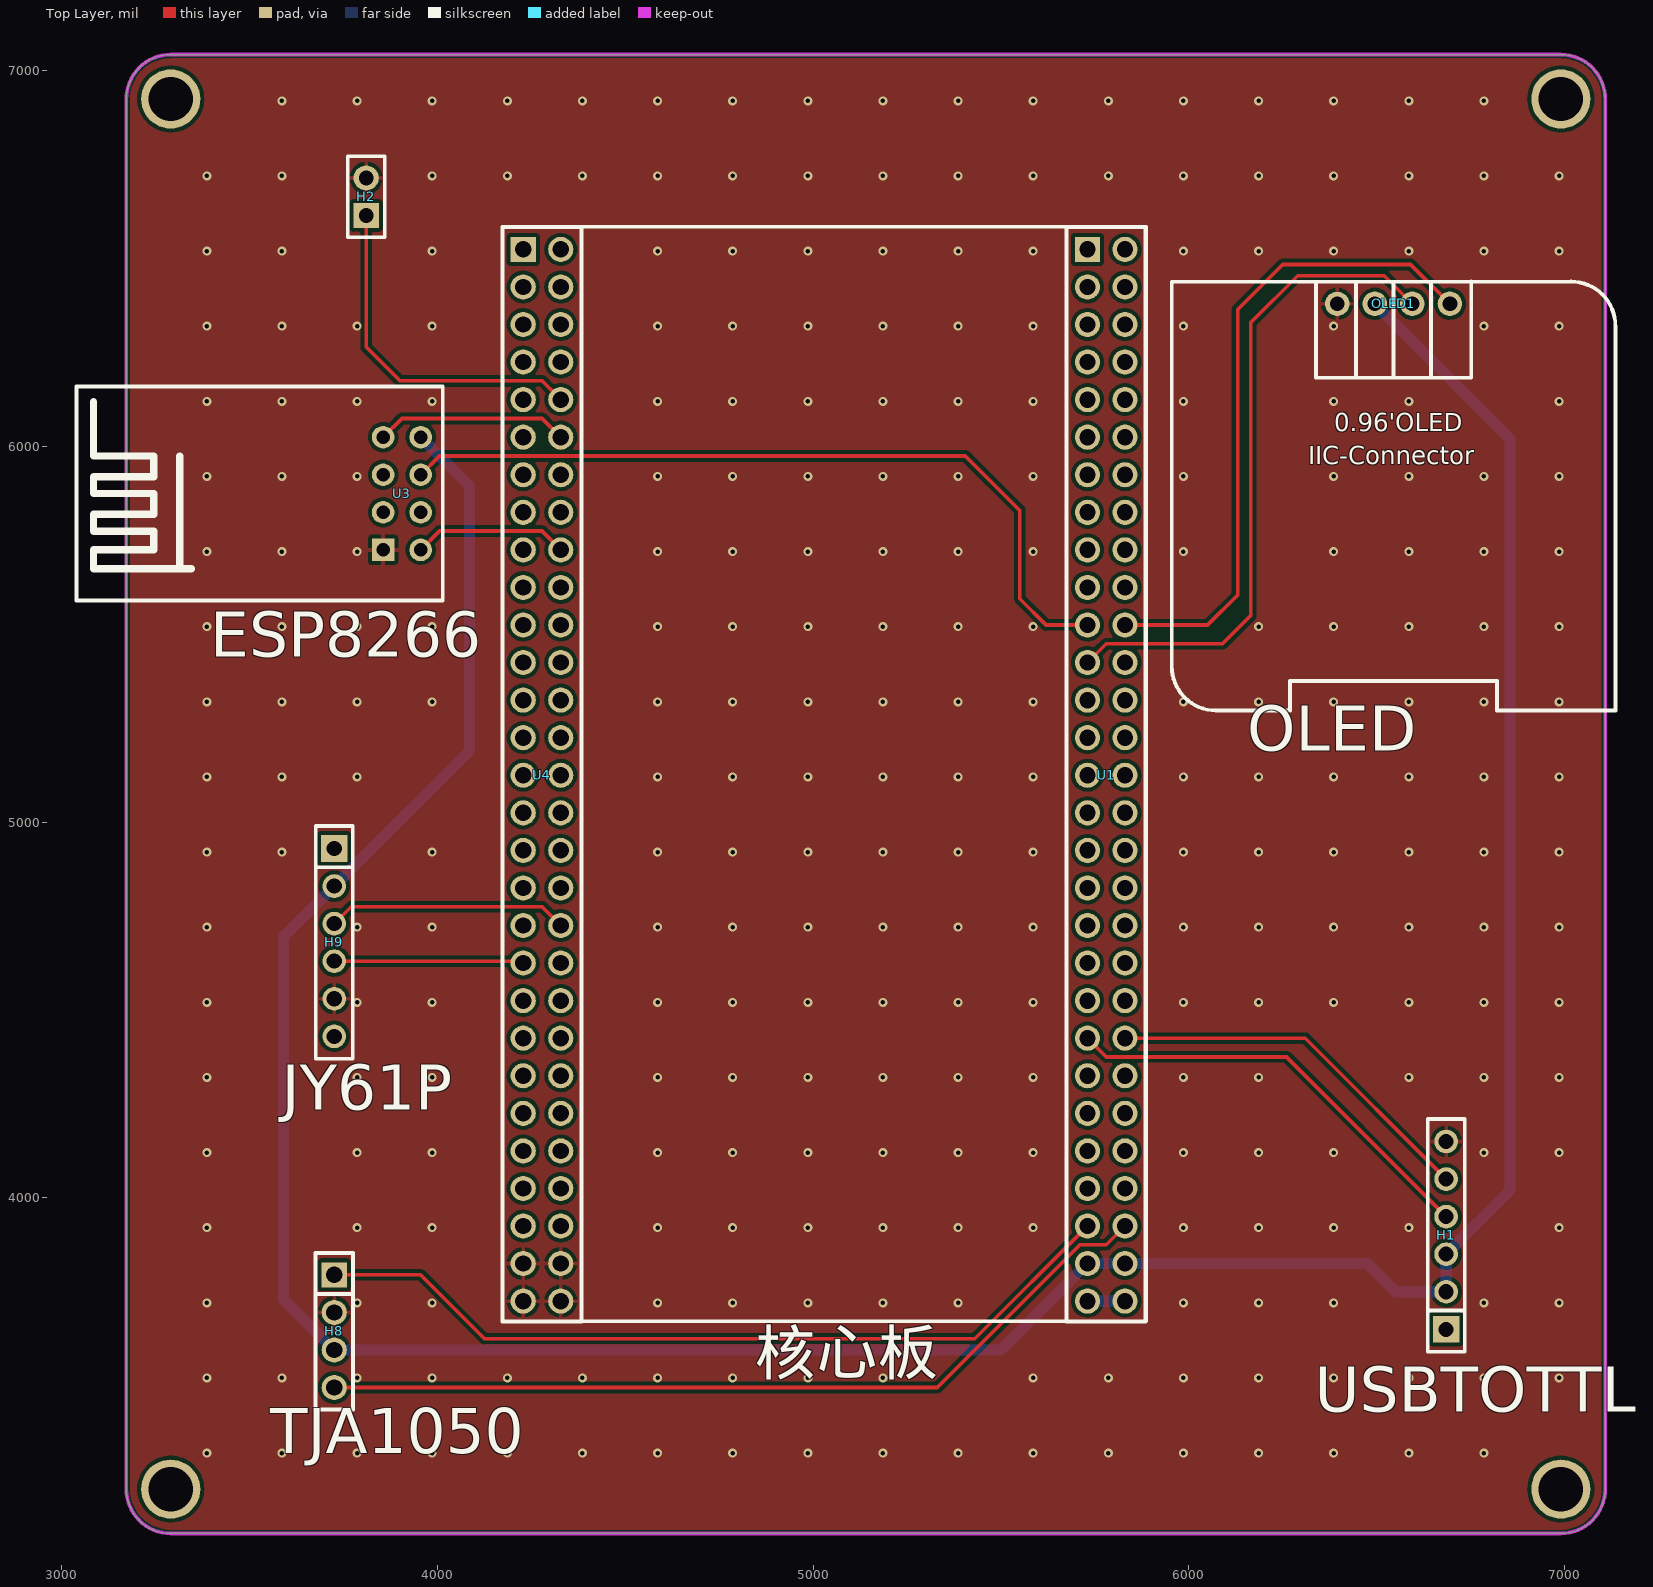
[diagram p0: Top Layer view]
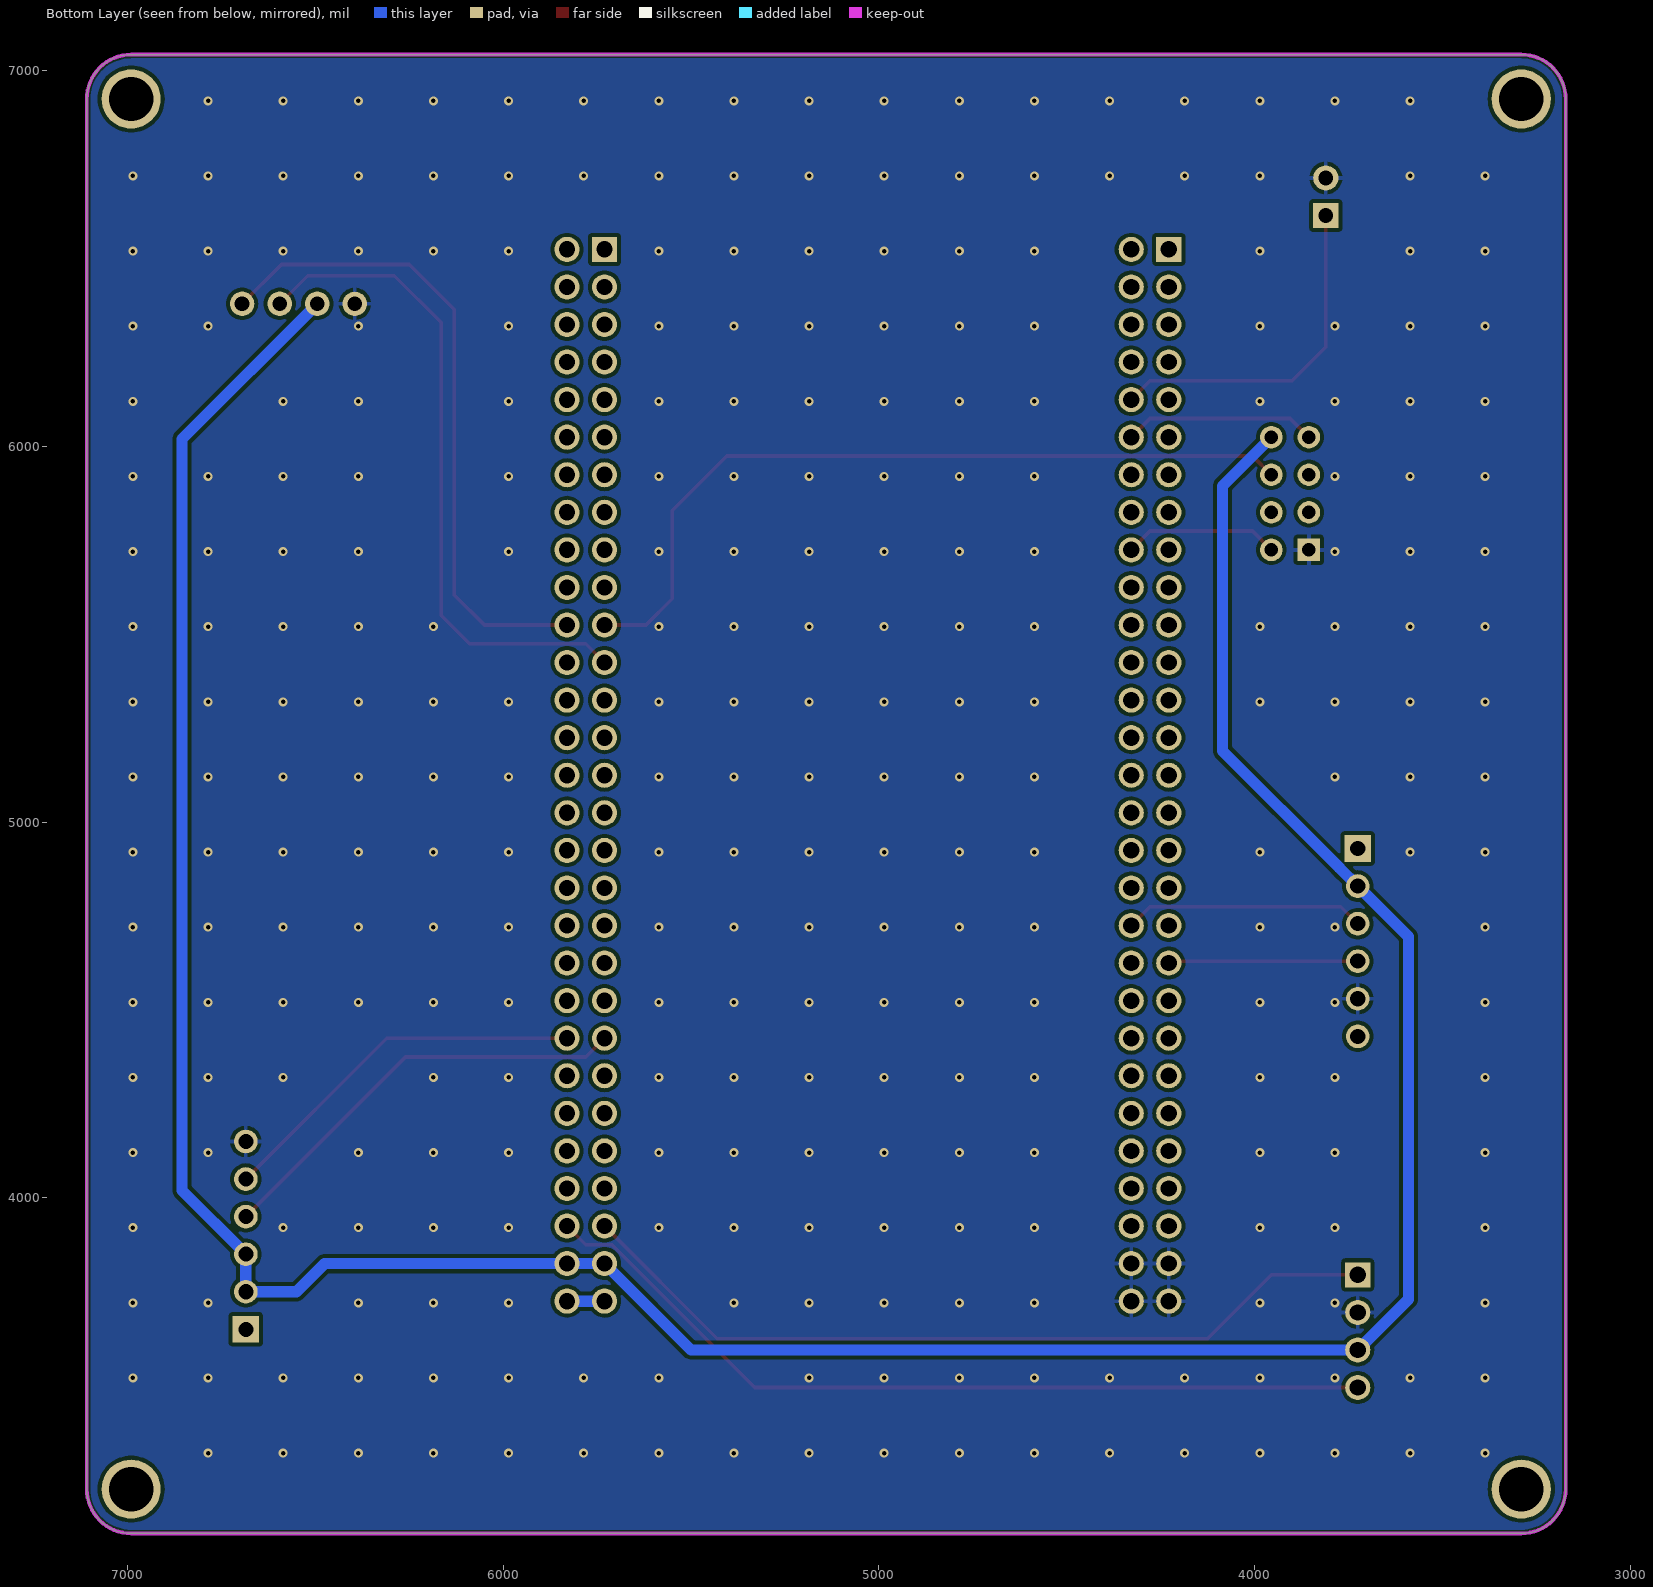
[diagram p1: Bottom Layer view, seen from below]
# Altium PCB MISC51816.pcbdoc
Units mil, origin at the board's own origin, x right, y up, seen from the top; angles counter-clockwise.
Board outline 3937.01 x 3937.01 mil, 2 copper layers (Top Layer, Bottom Layer), stack 62.206 mil thick; 8 components, 112 nets, 150 pads, 288 vias.

## Layer stack, top to bottom
Top Solder Mask Layer: solder mask 0.394, Dk 3.3
Top Layer: signal copper 1.379
Dielectric1: surface 59.449, FR4, Dk 4.5
Bottom Layer: signal copper 1.378
Bottom Solder Mask Layer: solder mask 0.394, Dk 3.3

## Board outline
6990.39,3106.5 ccw(c6990.39,3224.61) 7108.5,3224.61 7108.5,6925.39 ccw(c6990.39,6925.39) 6990.39,7043.5 3289.61,7043.5 ccw(c3289.61,6925.39) 3171.5,6925.39 3171.5,3224.61 ccw(c3289.61,3224.61) 3289.61,3106.5

## Design rules (kind name [scope] priority, off if disabled: settings)
BoardOutlineClearance copperThickness2oz_1 [All] p2 off: genericclearance=7.99 ignorepadtopadclearanceinfootprint=FALSE except(0: Arc-SplitContinuation Track-SplitContinuation SMDPad-SplitContinuation THPad-SplitContinuation Via-SplitContinuation Fill-SplitContinuation Region-SplitContinuation Poly-SplitContinuation Text-SplitContinuation Hole-SplitContinuation; 5.98: Arc-CutoutEdge Track-CutoutEdge SMDPad-CutoutEdge THPad-CutoutEdge Via-CutoutEdge Text-CutoutEdge; 6.89: Hole-OutlineEdge Hole-CutoutEdge; 10: Poly-OutlineEdge Poly-CutoutEdge; 11.81: Arc-OutlineEdge Track-OutlineEdge SMDPad-OutlineEdge THPad-OutlineEdge Via-OutlineEdge Fill-OutlineEdge Region-OutlineEdge Text-OutlineEdge Fill-CutoutEdge Region-CutoutEdge)
BoardOutlineClearance Plane_innerPlane_1 [All] p4 off: genericclearance=4.02 ignorepadtopadclearanceinfootprint=FALSE except(0: Arc-SplitContinuation Track-SplitContinuation SMDPad-SplitContinuation THPad-SplitContinuation Via-SplitContinuation Fill-SplitContinuation Region-SplitContinuation Poly-SplitContinuation Text-SplitContinuation Hole-SplitContinuation; 5.98: Arc-CutoutEdge Track-CutoutEdge SMDPad-CutoutEdge THPad-CutoutEdge Via-CutoutEdge Text-CutoutEdge; 6.89: Hole-OutlineEdge Hole-CutoutEdge; 10: Poly-OutlineEdge Poly-CutoutEdge; 11.81: Arc-OutlineEdge Track-OutlineEdge SMDPad-OutlineEdge THPad-OutlineEdge Via-OutlineEdge Fill-OutlineEdge Region-OutlineEdge Text-OutlineEdge Fill-CutoutEdge Region-CutoutEdge)
BoardOutlineClearance Copper_copperRegion_1 [All] p6 off: genericclearance=4.02 ignorepadtopadclearanceinfootprint=FALSE except(0: Arc-SplitContinuation Track-SplitContinuation SMDPad-SplitContinuation THPad-SplitContinuation Via-SplitContinuation Fill-SplitContinuation Region-SplitContinuation Poly-SplitContinuation Text-SplitContinuation Hole-SplitContinuation; 5.98: Arc-CutoutEdge Track-CutoutEdge SMDPad-CutoutEdge THPad-CutoutEdge Via-CutoutEdge Text-CutoutEdge; 6.89: Hole-OutlineEdge Hole-CutoutEdge; 10: Poly-OutlineEdge Poly-CutoutEdge; 11.81: Arc-OutlineEdge Track-OutlineEdge SMDPad-OutlineEdge THPad-OutlineEdge Via-OutlineEdge Fill-OutlineEdge Region-OutlineEdge Text-OutlineEdge Fill-CutoutEdge Region-CutoutEdge)
BoardOutlineClearance copperThickness1oz_1 [All] p8: genericclearance=4.02 ignorepadtopadclearanceinfootprint=FALSE except(0: Arc-SplitContinuation Track-SplitContinuation SMDPad-SplitContinuation THPad-SplitContinuation Via-SplitContinuation Fill-SplitContinuation Region-SplitContinuation Poly-SplitContinuation Text-SplitContinuation Hole-SplitContinuation; 5.98: Arc-CutoutEdge Track-CutoutEdge SMDPad-CutoutEdge THPad-CutoutEdge Via-CutoutEdge Text-CutoutEdge; 6.89: Hole-OutlineEdge Hole-CutoutEdge; 10: Poly-OutlineEdge Poly-CutoutEdge; 11.81: Arc-OutlineEdge Track-OutlineEdge SMDPad-OutlineEdge THPad-OutlineEdge Via-OutlineEdge Fill-OutlineEdge Region-OutlineEdge Text-OutlineEdge Fill-CutoutEdge Region-CutoutEdge)
Clearance copperThickness2oz [All] p1 off: gap=7.99 ignorepadtopadclearanceinfootprint=FALSE except(5.98: SMDPad-Track SMDPad-SMDPad THPad-Track SMDPad-THPad THPad-THPad Track-Via SMDPad-Via THPad-Via Via-Via Fill-SMDPad Region-SMDPad Fill-THPad Region-THPad Fill-Via Region-Via Fill-Fill Fill-Region Region-Region Arc-Track Arc-SMDPad Arc-THPad Arc-Via Fill-Arc Region-Arc Arc-Arc Text-Track SMDPad-Text Text-THPad Text-Via Fill-Text Region-Text Arc-Text Text-Text; 6.89: Hole-Track Hole-SMDPad Hole-THPad Hole-Via Fill-Hole Region-Hole Hole-Arc Hole-Text; 10: Poly-Track Poly-SMDPad Poly-THPad Poly-Via Poly-Fill Poly-Region Poly-Poly Poly-Arc Poly-Text Poly-Hole; 11.81: Fill-Track Region-Track)
Clearance Plane_innerPlane [All] p3 off: gap=4.02 ignorepadtopadclearanceinfootprint=FALSE except(5.98: SMDPad-Track SMDPad-SMDPad THPad-Track SMDPad-THPad THPad-THPad Track-Via SMDPad-Via THPad-Via Via-Via Fill-SMDPad Region-SMDPad Fill-THPad Region-THPad Fill-Via Region-Via Fill-Fill Fill-Region Region-Region Arc-Track Arc-SMDPad Arc-THPad Arc-Via Fill-Arc Region-Arc Arc-Arc Text-Track SMDPad-Text Text-THPad Text-Via Fill-Text Region-Text Arc-Text Text-Text; 6.89: Hole-Track Hole-SMDPad Hole-THPad Hole-Via Fill-Hole Region-Hole Hole-Arc Hole-Text; 10: Poly-Track Poly-SMDPad Poly-THPad Poly-Via Poly-Fill Poly-Region Poly-Poly Poly-Arc Poly-Text Poly-Hole; 11.81: Fill-Track Region-Track)
Clearance Copper_copperRegion [All] p5 off: gap=4.02 ignorepadtopadclearanceinfootprint=FALSE except(5.98: SMDPad-Track SMDPad-SMDPad THPad-Track SMDPad-THPad THPad-THPad Track-Via SMDPad-Via THPad-Via Via-Via Fill-SMDPad Region-SMDPad Fill-THPad Region-THPad Fill-Via Region-Via Fill-Fill Fill-Region Region-Region Arc-Track Arc-SMDPad Arc-THPad Arc-Via Fill-Arc Region-Arc Arc-Arc Text-Track SMDPad-Text Text-THPad Text-Via Fill-Text Region-Text Arc-Text Text-Text; 6.89: Hole-Track Hole-SMDPad Hole-THPad Hole-Via Fill-Hole Region-Hole Hole-Arc Hole-Text; 10: Poly-Track Poly-SMDPad Poly-THPad Poly-Via Poly-Fill Poly-Region Poly-Poly Poly-Arc Poly-Text Poly-Hole; 11.81: Fill-Track Region-Track)
Clearance copperThickness1oz [All] p7: gap=4.02 ignorepadtopadclearanceinfootprint=FALSE except(5.98: SMDPad-Track SMDPad-SMDPad THPad-Track SMDPad-THPad THPad-THPad Track-Via SMDPad-Via THPad-Via Via-Via Fill-SMDPad Region-SMDPad Fill-THPad Region-THPad Fill-Via Region-Via Fill-Fill Fill-Region Region-Region Arc-Track Arc-SMDPad Arc-THPad Arc-Via Fill-Arc Region-Arc Arc-Arc Text-Track SMDPad-Text Text-THPad Text-Via Fill-Text Region-Text Arc-Text Text-Text; 6.89: Hole-Track Hole-SMDPad Hole-THPad Hole-Via Fill-Hole Region-Hole Hole-Arc Hole-Text; 10: Poly-Track Poly-SMDPad Poly-THPad Poly-Via Poly-Fill Poly-Region Poly-Poly Poly-Arc Poly-Text Poly-Hole; 11.81: Fill-Track Region-Track)
DiffPairsRouting differentialPair [All] p1: maxlimit=6 minlimit=6 mostfreqgap=6 toplayer_minwidth=5 toplayer_prefwidth=10 toplayer_maxwidth=100 toplayer_mingap=6 toplayer_prefgap=6 toplayer_maxgap=6 bottomlayer_minwidth=5 bottomlayer_prefwidth=10 bottomlayer_maxwidth=100 bottomlayer_mingap=6 bottomlayer_prefgap=6 bottomlayer_maxgap=6 maxuncoupledlength=10
HoleToHoleClearance otherClearance [All] p1: gap=11.81 allowstackedmicrovias=TRUE
Length netLength [All] p1: minlimit=0 maxlimit=0
PasteMaskExpansion pasteMaskExpansion [All] p1: expansion=0
PlaneConnect innerPlane [All] p1: planeconnectstyle=Relief reliefexpansion=20 reliefentries=4 reliefconductorwidth=10 reliefairgap=10
PolygonConnect copperRegion [All] p1: connectstyle=Relief reliefconductorwidth=10 reliefentries=4 polygonreliefangle="90 Angle" airgapwidth=10 via.connectstyle=Relief via.reliefconductorwidth=10 via.reliefentries=4 via.polygonreliefangle="90 Angle" via.airgapwidth=10
RoutingVias viaSize [All] p1: holewidth=12.01 width=24.02 viastyle="Through Hole" minholewidth=11.81 minwidth=19.68 maxholewidth=248.03 maxwidth=393.7
SolderMaskExpansion solderMaskExpansion [IsVia] p1: expansion=-1000 istentingtop=TRUE
SolderMaskExpansion solderMaskExpansion [All] p2: expansion=2.01 istentingtop=FALSE
Width copperThickness2oz_2 [All] p1 off: maxlimit=100 minlimit=8 preferedwidth=10
Width copperThickness1oz_2 [All] p2: maxlimit=100 minlimit=5 preferedwidth=30

## Components (designator, comment, footprint, x,y, rotation, side; value= is the part's Value field where it differs from the comment)
H1 "" HDR-TH_6P-P2.54-V-F 6685,3900 r90 top
H2 "" HDR-TH_2P-P2.54-V-F 3810,6665 r90 top
H8 "" HDR-TH_4P-P2.54-V-F 3725,3645 r270 top
H9 "" HDR-TH_6P-P2.54-V-F 3725,4680 r270 top
OLED1 "" 0.96OLED_4P 6545,6380 r0 top
U1 "XDFH-0254-2*30P" CONN-TH_60P-P2.54_LX_XDFH-0254-2X30P 5780,5075 r270 top
U3 "ESP8266-01S" WIFIM-TH_ESP8266-01S 3905,5875 r90 top
U4 "XDFH-0254-2*30P" CONN-TH_60P-P2.54_LX_XDFH-0254-2X30P 4278.02,5075 r270 top

## Footprints (in the part's own frame and the unit in brackets; to place one, negate y for a bottom-side part, rotate by r counter-clockwise, add the part's x,y. Pads: shape width x height; smd on the part's side, far side on the other; paste and mask are expansions set on the pad)
0.96OLED_4P [mm]
  round 1.65 hole 1 copper offset 0,0: 1(-3.81,-0.001) 2(-1.27,0.002) 3(1.27,0.002) 4(3.81,0.002)
  silkscreen extent -15,-27.5 15,1.5
CONN-TH_60P-P2.54_LX_XDFH-0254-2X30P [mm]
  rect 1.7x1.7 hole 1.1 paste+0 mask+0.05: 1(-36.83,-1.27)
  round 1.7 hole 1.1 paste+0 mask+0.05: 2(-36.83,1.27) 3(-34.29,-1.27) 4(-34.29,1.27) 5(-31.75,-1.27) 6(-31.75,1.27) 7(-29.21,-1.27) 8(-29.21,1.27) 9(-26.67,-1.27) 10(-26.67,1.27) 11(-24.13,-1.27) 12(-24.13,1.27) 13(-21.59,-1.27) 14(-21.59,1.27) 15(-19.05,-1.27) 16(-19.05,1.27) 17(-16.51,-1.27) 18(-16.51,1.27) 19(-13.97,-1.27) 20(-13.97,1.27) 21(-11.43,-1.27) 22(-11.43,1.27) 23(-8.89,-1.27) 24(-8.89,1.27) 25(-6.35,-1.27) 26(-6.35,1.27) 27(-3.81,-1.27) 28(-3.81,1.27) 29(-1.27,-1.27) 30(-1.27,1.27) 31(1.27,-1.27) 32(1.27,1.27) 33(3.81,-1.27) 34(3.81,1.27) 35(6.35,-1.27) 36(6.35,1.27) 37(8.89,-1.27) 38(8.89,1.27) 39(11.43,-1.27) 40(11.43,1.27) 41(13.97,-1.27) 42(13.97,1.27) 43(16.51,-1.27) 44(16.51,1.27) 45(19.05,-1.27) 46(19.05,1.27) 47(21.59,-1.27) 48(21.59,1.27) 49(24.13,-1.27) 50(24.13,1.27) 51(26.67,-1.27) 52(26.67,1.27) 53(29.21,-1.27) 54(29.21,1.27) 55(31.75,-1.27) 56(31.75,1.27) 57(34.29,-1.27) 58(34.29,1.27)
  silkscreen extent -38.32,-2.69 35.67,2.67
HDR-TH_2P-P2.54-V-F [mm]
  rect 1.7x1.7 hole 1: 1(-1.27,0)
  round 1.7 hole 1: 2(1.27,0)
  silkscreen extent -2.74,-1.25 2.74,1.25
HDR-TH_4P-P2.54-V-F [mm]
  rect 1.7x1.7 hole 1.1: 1(-3.81,0)
  round 1.7 hole 1.1: 2(-1.27,0) 3(1.27,0) 4(3.81,0)
  silkscreen extent -5.29,-1.27 5.29,1.27
HDR-TH_6P-P2.54-V-F [mm]
  rect 1.8x1.8 hole 1.02: 1(-6.35,0)
  round 1.6 hole 1.02: 2(-3.81,0) 3(-1.27,0) 4(1.27,0) 5(3.81,0) 6(6.35,0)
  silkscreen extent -7.87,-1.25 7.87,1.25
WIFIM-TH_ESP8266-01S [mil]
  rect 60x60 hole 36 paste+0 mask+1.97: 1(-150,50)
  round 60 hole 36 paste+0 mask+1.97: 2(-50,50) 3(50,50) 4(150,50) 5(-150,-50) 6(-50,-50) 7(50,-50) 8(150,-50)
  silkscreen extent -285,-109 285,866

## Free pads (board coordinates)
  round 157.48 hole 118.11: 1(3289.61,6925.39) 1(3289.61,3224.61) 1(6990.39,6925.39) 1(6990.39,3224.61)

## Via types
v1: diameter 24.02, hole 12, Top Layer to Bottom Layer, 288 vias

## Nets (pads, with @x,y where several pads share a name; then routed paths per layer and width w, separated by ;. In a path a pad name is that pad's centre, name@x,y a point inside that pad or via, vN(x,y) a via of type N, cw(c..) or ccw(c..) an arc to the next point about the centre after c; other vN are vias at no path point)
5V: U1.57 U1.58 | length 100
  Bottom Layer w30: U1.57 U1.58
+5V: H1.1
A0: H2.1 U4.10 | length 926
  Top Layer w10: H2.1 3810,6265 3900,6175 4278.02,6175 U4.10
A1: U4.9
A2: U3.4 U4.12 | length 514.4
  Top Layer w10: U3.4 3905,6075 4278.02,6075 U4.12
A3: U3.5 U4.18 | length 414.4
  Top Layer w10: U3.5 4005,5775 4278.02,5775 U4.18
A4: U4.17
A5: U4.20
A6: U4.19
A7: U4.22
A8: U1.42
A9: H1.5 U1.44 | length 1010.3
  Top Layer w10: U1.44 6310,4425 H1.5
A10: H1.4 U1.43 | length 1151.8
  Top Layer w10: U1.43 5780,4375 6260,4375 H1.4
A11: H8.4 U1.54 | length 2283.1
  Top Layer w10: H8.4 5330,3495 5710,3875 5780,3875 U1.54
A12: H8.1 U1.53 | length 2199.7
  Top Layer w10: H8.1 3955,3795 4125,3625 5430,3625 U1.53
A15: U1.9
B0: U4.16
B1: U4.13
B2: U4.24
B3: U1.26
B4: U1.25
B5: U1.24
B6: OLED1.3 U1.23 | length 1779.6
  Top Layer w10: U1.23 5780,5475 6090,5475 6165,5550 6165,6330 6290,6455 6520.05,6455 OLED1.3@6595,6380.05
B7: OLED1.4 U1.22 | length 1751.3
  Top Layer w10: U1.22 6050,5525 6130,5605 6130,6365 6250,6485 6590.05,6485 OLED1.4@6695,6380.05
B8: U1.21 U3.7 | length 2119.8
  Top Layer w10: U3.7 4005,5975 5405,5975 5550,5830 5550,5595 5620,5525 U1.21
B9: U1.20
B10: H9.3 U4.38 | length 642.4
  Top Layer w10: H9.3 3770,4775 4278.02,4775 U4.38
B11: H9.4 U4.39 | length 505.1
  Top Layer w10: H9.4 4223.02,4630 U4.39
B12: U4.45
B13: U4.46
B14: U4.47
B15: U4.48
C0: U4.3
C1: U4.4
C2: U4.1
C3: U4.2
C4: U4.21
C5: U4.15
C6: U1.47
C7: U1.48
C8: U1.45
C9: U1.46
C10: U1.41
C11: U1.40
C12: U1.39
C13: U1.8
D0: U1.38
D1: U1.37
D2: U1.36
D3: U1.35
D4: U1.34
D5: U1.33
D6: U1.32
D7: U1.31
D8: U4.49
D9: U4.50
D10: U4.51
D11: U4.52
D12: U4.53
D13: U4.54
D14: U4.44
D15: U4.43
E0: U1.18
E1: U1.19
E2: U1.14
E3: U1.13
E4: U1.12
E5: U1.11
E6: U1.10
E7: U4.30
E8: U4.29
E9: U4.31
E10: U4.32
E11: U4.33
E12: U4.34
E13: U4.35
E13': U4.14
E14: U4.36
E15: U4.37
F0: U1.7
F1: U1.6
F2: U1.5
F3: U1.4
F4: U1.3
F5: U1.2
F6: U1.1
F7: U4.7
F8: U4.8
F9: U4.5
F10: U4.6
F11: U4.23
F12: U4.26
F14: U4.11
F15: U4.25
G0: U4.28
G1: U4.27
G2: U4.42
G3: U4.41
G4: U4.40
G5: U1.51
G6: U1.52
G7: U1.49
G8: U1.50
G9: U1.30
G10: U1.29
G11: U1.28
G12: U1.15
G13: U1.16
G14: U1.17
G15: U1.27
GND: H1.6 H2.2 H8.2 H9.5 OLED1.1 U3.1 U4.55 U4.56 U4.57 U4.58
  other v1: 3385.6,3320.6 3585.6,3320.6 3785.6,3320.6 3985.6,3320.6 4185.6,3320.6 4385.6,3320.6 4585.6,3320.6 4785.6,3320.6 4985.6,3320.6 5185.6,3320.6 5385.6,3320.6 5585.6,3320.6 5785.6,3320.6 5985.6,3320.6 6185.6,3320.6 6385.6,3320.6 6585.6,3320.6 6785.6,3320.6 3385.6,3520.6 3585.6,3520.6 3785.6,3520.6 3985.6,3520.6 4185.6,3520.6 4385.6,3520.6 4585.6,3520.6 4785.6,3520.6 4985.6,3520.6 5185.6,3520.6 5585.6,3520.6 5785.6,3520.6 5985.6,3520.6 6185.6,3520.6 6385.6,3520.6 6585.6,3520.6 6785.6,3520.6 6985.6,3520.6 3385.6,3720.6 3785.6,3720.6 3985.6,3720.6 4585.6,3720.6 4785.6,3720.6 4985.6,3720.6 5185.6,3720.6 5385.6,3720.6 5985.6,3720.6 6185.6,3720.6 6385.6,3720.6 6785.6,3720.6 6985.6,3720.6 3385.6,3920.6 3785.6,3920.6 3985.6,3920.6 4585.6,3920.6 4785.6,3920.6 4985.6,3920.6 5185.6,3920.6 5385.6,3920.6 5585.6,3920.6 5985.6,3920.6 6185.6,3920.6 6385.6,3920.6 6585.6,3920.6 6985.6,3920.6 3385.6,4120.6 3785.6,4120.6 3985.6,4120.6 4585.6,4120.6 4785.6,4120.6 4985.6,4120.6 5185.6,4120.6 5385.6,4120.6 5585.6,4120.6 5985.6,4120.6 6185.6,4120.6 6385.6,4120.6 6785.6,4120.6 6985.6,4120.6 3385.6,4320.6 3785.6,4320.6 3985.6,4320.6 4585.6,4320.6 4785.6,4320.6 4985.6,4320.6 5185.6,4320.6 5385.6,4320.6 5585.6,4320.6 5985.6,4320.6 6185.6,4320.6 6585.6,4320.6 6785.6,4320.6 6985.6,4320.6 3385.6,4520.6 3785.6,4520.6 3985.6,4520.6 4585.6,4520.6 4785.6,4520.6 4985.6,4520.6 5185.6,4520.6 5385.6,4520.6 5585.6,4520.6 5985.6,4520.6 6185.6,4520.6 6385.6,4520.6 6585.6,4520.6 6785.6,4520.6 6985.6,4520.6 3385.6,4720.6 3785.6,4720.6 3985.6,4720.6 4585.6,4720.6 4785.6,4720.6 4985.6,4720.6 5185.6,4720.6 5385.6,4720.6 5585.6,4720.6 5985.6,4720.6 6185.6,4720.6 6385.6,4720.6 6585.6,4720.6 6785.6,4720.6 6985.6,4720.6 3385.6,4920.6 3585.6,4920.6 3985.6,4920.6 4585.6,4920.6 4785.6,4920.6 4985.6,4920.6 5185.6,4920.6 5385.6,4920.6 5585.6,4920.6 5985.6,4920.6 6185.6,4920.6 6385.6,4920.6 6585.6,4920.6 6785.6,4920.6 6985.6,4920.6 3385.6,5120.6 3585.6,5120.6 3785.6,5120.6 4585.6,5120.6 4785.6,5120.6 4985.6,5120.6 5185.6,5120.6 5385.6,5120.6 5585.6,5120.6 5985.6,5120.6 6185.6,5120.6 6385.6,5120.6 6585.6,5120.6 6785.6,5120.6 6985.6,5120.6 3385.6,5320.6 3585.6,5320.6 3785.6,5320.6 3985.6,5320.6 4585.6,5320.6 4785.6,5320.6 4985.6,5320.6 5185.6,5320.6 5385.6,5320.6 5585.6,5320.6 5985.6,5320.6 6185.6,5320.6 6385.6,5320.6 6585.6,5320.6 6785.6,5320.6 6985.6,5320.6 3385.6,5520.6 3585.6,5520.6 3785.6,5520.6 3985.6,5520.6 4585.6,5520.6 4785.6,5520.6 4985.6,5520.6 5185.6,5520.6 5385.6,5520.6 5585.6,5520.6 6185.6,5520.6 6385.6,5520.6 6585.6,5520.6 6785.6,5520.6 6985.6,5520.6 3385.6,5720.6 3585.6,5720.6 3785.6,5720.6 4585.6,5720.6 4785.6,5720.6 4985.6,5720.6 5185.6,5720.6 5385.6,5720.6 5585.6,5720.6 5985.6,5720.6 6385.6,5720.6 6585.6,5720.6 6785.6,5720.6 6985.6,5720.6 3385.6,5920.6 3585.6,5920.6 3785.6,5920.6 4585.6,5920.6 4785.6,5920.6 4985.6,5920.6 5185.6,5920.6 5385.6,5920.6 5585.6,5920.6 5985.6,5920.6 6385.6,5920.6 6585.6,5920.6 6785.6,5920.6 6985.6,5920.6 3385.6,6120.6 3585.6,6120.6 3785.6,6120.6 3985.6,6120.6 4585.6,6120.6 4785.6,6120.6 4985.6,6120.6 5185.6,6120.6 5385.6,6120.6 5585.6,6120.6 5985.6,6120.6 6385.6,6120.6 6585.6,6120.6 6985.6,6120.6 3385.6,6320.6 3585.6,6320.6 3785.6,6320.6 3985.6,6320.6 4585.6,6320.6 4785.6,6320.6 4985.6,6320.6 5185.6,6320.6 5385.6,6320.6 5585.6,6320.6 5985.6,6320.6 6385.6,6320.6 6785.6,6320.6 6985.6,6320.6 3385.6,6520.6 3585.6,6520.6 3985.6,6520.6 4585.6,6520.6 4785.6,6520.6 4985.6,6520.6 5185.6,6520.6 5385.6,6520.6 5585.6,6520.6 5985.6,6520.6 6185.6,6520.6 6385.6,6520.6 6585.6,6520.6 6785.6,6520.6 6985.6,6520.6 3385.6,6720.6 3585.6,6720.6 3985.6,6720.6 4185.6,6720.6 4385.6,6720.6 4585.6,6720.6 4785.6,6720.6 4985.6,6720.6 5185.6,6720.6 5385.6,6720.6 5585.6,6720.6 5785.6,6720.6 5985.6,6720.6 6185.6,6720.6 6385.6,6720.6 6585.6,6720.6 6785.6,6720.6 6985.6,6720.6 3585.6,6920.6 3785.6,6920.6 3985.6,6920.6 4185.6,6920.6 4385.6,6920.6 4585.6,6920.6 4785.6,6920.6 4985.6,6920.6 5185.6,6920.6 5385.6,6920.6 5585.6,6920.6 5785.6,6920.6 5985.6,6920.6 6185.6,6920.6 6385.6,6920.6 6585.6,6920.6 6785.6,6920.6
VCC: H1.2 H1.3 H8.3 H9.2 OLED1.2 U1.55 U1.56 U3.8 | length 8680.8
  Bottom Layer w30: U3.8 4085,5895 4085,5190 3777.82,4882.82 cw(c3760.43,4894.57) 3772.18,4877.18 H9.2 3590,4695 3590,3730 H8.3 5500,3595 U1.55 U1.56 6475,3825 6550,3750 H1.2 H1.3 6855,4020 6855,6020.05 OLED1.2@6495,6380.05
pads on no net: H9.1 H9.6 U3.2 U3.3 U3.6

## Polygon pours and split planes (outlines as drawn)
GND on Bottom Layer (solid, remove dead copper, pour order 2): 3100,7165 3100,3000 7275,3000 7275,7165
GND on Top Layer (solid, remove dead copper, pour order 0): 3000,7145 3000,3075 7385,3075 7385,7145

## Keep-outs
Board Outline Layer:
  the board outline again, w10

## Silkscreen, mask and mechanical layers (free items; w line width, h text height)
Top Silkscreen Layer:
  lines w10: 4173.03,3671.61 4173.03,6585 5885.63,6585 5885.63,3671.61 4173.03,3671.61
  text "ESP8266" at 3395,5440 h120
  text "OLED" at 6155,5190 h120
  text "JY61P" at 3585,4235 h120
  text "核心板" at 4845,3530 h120
  text "USBTOTTL" at 6335,3430 h120
  text "TJA1050" at 3555,3320 h120